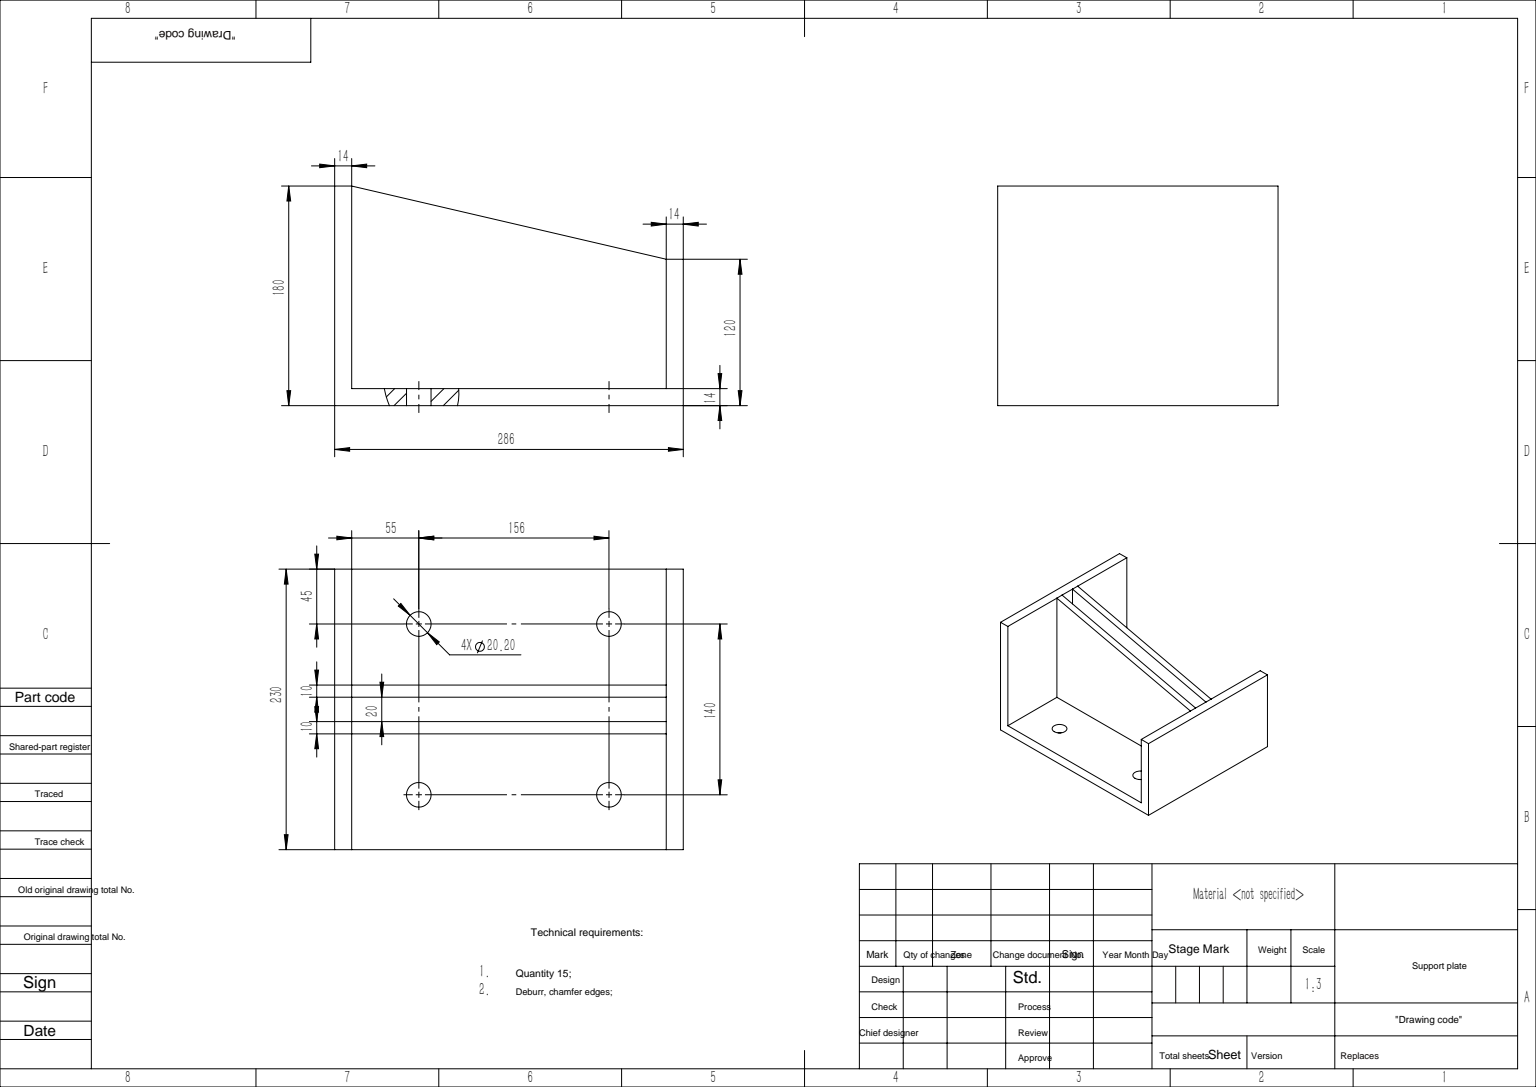
SolidWorks part; units mm, degrees
ref_plane "前视基准面" through (0, 0, 0) normal (0, 0, 1) x (1, 0, 0)
ref_plane "上视基准面" through (0, 0, 0) normal (0, 1, 0) x (1, 0, 0)
ref_plane "右视基准面" through (0, 0, 0) normal (1, 0, 0) x (0, 0, -1)
sketch "草图1" plane through (0, 0, 0) normal (0, 0, 1) x (1, 0, 0)
  line L0 (0, 0) -> (0, 254.1548) construction
  line L1 (-143, 180) -> (-129, 180)
  line L2 (-143, 180) -> (-143, 0)
  line L3 (-143, 0) -> (143, 0)
  line L4 (143, 120) -> (143, 0)
  line L5 (-129, 180) -> (-129, 14)
  line L6 (-129, 14) -> (129, 14)
  line L7 (129, 14) -> (129, 120)
  line L8 (129, 120) -> (143, 120)
  dimension "D1" = 286
  dimension "D2" = 120
  dimension "D3" = 14
  dimension "D4" = 14
  dimension "D5" = 180
extrude "凸台-拉伸1" add sketch "草图1" along normal mid plane 230
sketch "草图2" plane through (0, 0, 0) normal (0, 0, 1) x (1, 0, 0)
  line L0 (129, 120) -> (129, 14) construction
  line L2 (129, 14) -> (-129, 14) construction
  line L3 (-129, 14) -> (-129, 180) construction
  line L4 (129, 120) -> (129, 14)
  line L5 (129, 14) -> (-129, 14)
  line L6 (-129, 14) -> (-129, 180)
  line L7 (-129, 180) -> (129, 120)
extrude "凸台-拉伸2" add sketch "草图2" against normal blind 10 from offset 10 offset against normal yes
sketch "草图3" plane through (0, 0, 0) normal (0, 0, 1) x (1, 0, 0)
  line L3 (-129, 180) -> (-129, 14)
  line L4 (-129, 14) -> (129, 14)
  line L5 (129, 120) -> (-129, 180)
  line L6 (-129, 180) -> (-129, 14)
  line L7 (-129, 14) -> (129, 14)
  line L8 (129, 120) -> (-129, 180)
  line L10 (129, 14) -> (129, 120)
  line L11 (129, 14) -> (129, 120)
  dimension "D1" = 0
extrude "凸台-拉伸3" add sketch "草图3" along normal blind 10 from offset 10
sketch "草图4" plane through (0, 14, 0) normal (0, 1, 0) x (1, 0, 0)
  line L0 (-129, -115) -> (-129, -20) construction
  line L2 (129, -115) -> (-129, -115) construction
  circle A0 centre (-74, -70) radius 10.1
  dimension "D1" = 20.2
  dimension "D2" = 55
  dimension "D3" = 45
extrude "切除-拉伸1" cut sketch "草图4" against normal through all
pattern_linear "阵列(线性)1" count 2 spacing 156 along (1, 0, 0) count 2 spacing 140 along (0, 0, -1) of "切除-拉伸1"
